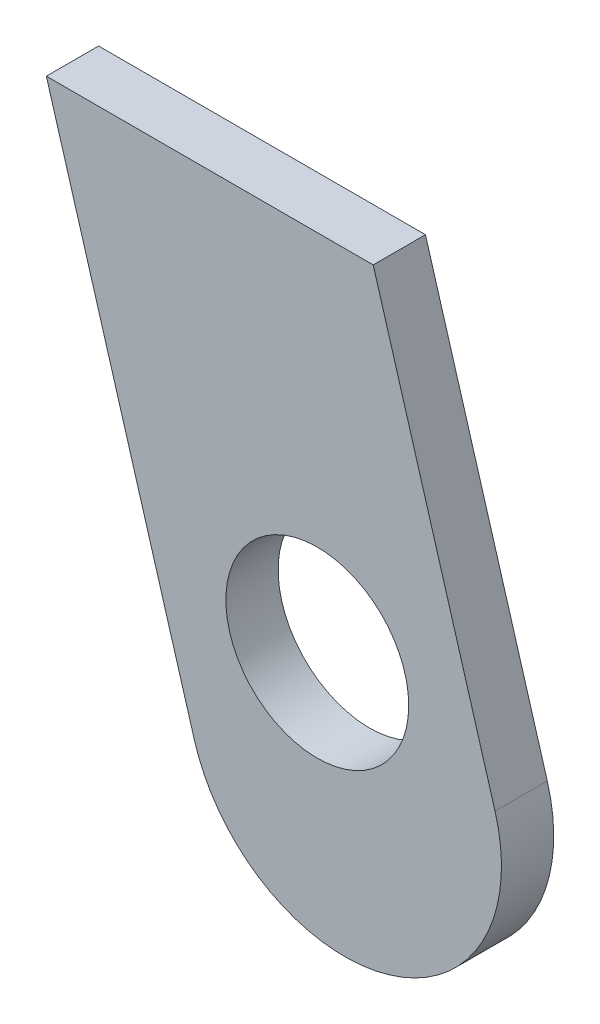
from build123d import *

# Parameters (mm, degrees)
SKETCH_2_R      = 17.5
EXTRUDE_1_DEPTH = 10


with BuildPart() as part:
    # 草图2 → 凸台-拉伸1 (new body)
    with BuildSketch(Plane.XY):
        with BuildLine():
            Line((507.065379812, -222.122666991), (535.409266278, -318.021697747))
            ThreePointArc((535.409266278, -318.021697747), (572.682141445, -338.288241034), (592.948684732, -301.015365867))
            Line((592.948684732, -301.015365867), (569.631184207, -222.122666991))
            Line((569.631184207, -222.122666991), (507.065379812, -222.122666991))
        make_face()
        with Locations((558.927759659, -291.75150785)):
            Circle(SKETCH_2_R, mode=Mode.SUBTRACT)
    extrude(amount=-EXTRUDE_1_DEPTH)


solid = part.part
